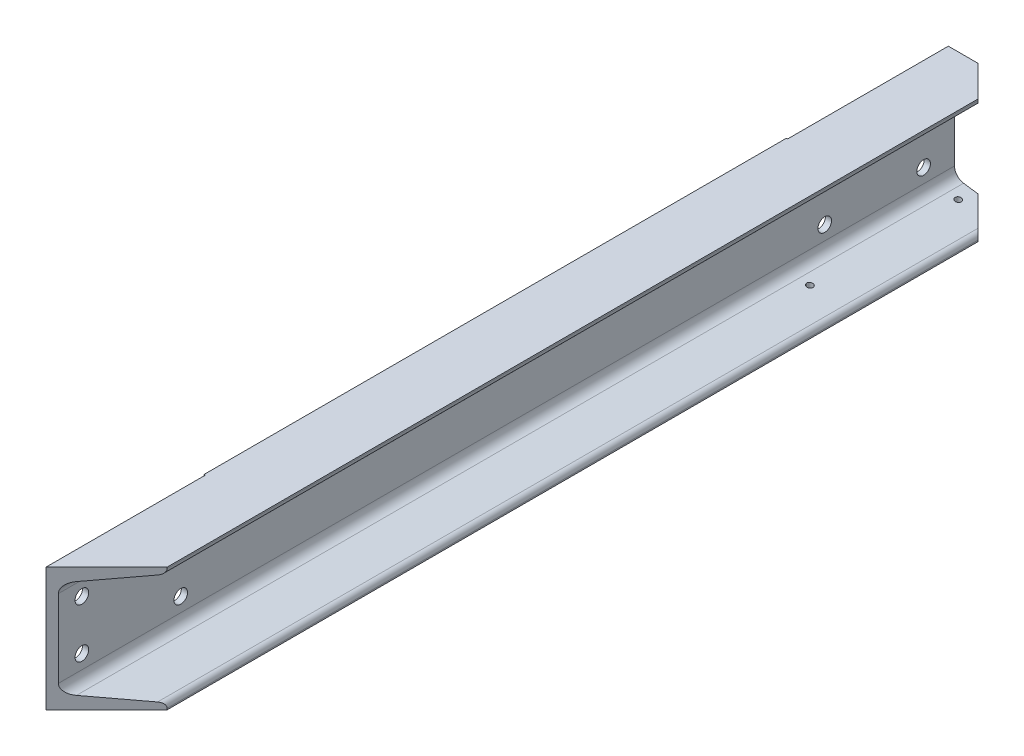
SolidWorks part; units mm, degrees
material "1023 carbon steel plate (SS)"
ref_plane "Front Plane" through (0, 0, 0) normal (0, 0, 1) x (1, 0, 0)
ref_plane "Top Plane" through (0, 0, 0) normal (0, 1, 0) x (1, 0, 0)
ref_plane "Right Plane" through (0, 0, 0) normal (1, 0, 0) x (0, 0, -1)
sketch "Sketch1" plane through (0, 0, 0) normal (0, 0, 1) x (1, 0, 0)
  line L0 (0, 0) -> (0, -100)
  line L1 (0, -100) -> (50, -100)
  line L2 (0, 0) -> (50, 0)
  line L3 (50, 0) -> (50, -1.0747)
  line L4 (50, -100) -> (50, -98.9253)
  line L5 (46.1263, -5.5309) -> (13.317, -10.1419)
  line L6 (6, -18.5592) -> (6, -81.4408)
  line L7 (13.317, -89.8581) -> (46.1263, -94.4691)
  line L8 (25, 0) -> (25, -8.5) construction
  line L9 (25, -100) -> (25, -91.5) construction
  arc A0 (6, -81.4408) -> (13.317, -89.8581) centre (14.5, -81.4408) ccw
  arc A1 (13.317, -10.1419) -> (6, -18.5592) centre (14.5, -18.5592) ccw
  arc A2 (50, -98.9253) -> (46.1263, -94.4691) centre (45.5, -98.9253) ccw
  arc A3 (50, -1.0747) -> (46.1263, -5.5309) centre (45.5, -1.0747) cw
  dimension "D8" = 8.5
  dimension "D9" = 4.5
  dimension "D1" = 100
  dimension "D2" = 50
  dimension "D3" = 50
  dimension "D4" = 6
  dimension "D5" = 8.5
  dimension "D6" = 8.5
  dimension "D7" = 98
extrude "Boss-Extrude1" add sketch "Sketch1" along normal blind 750
sketch "Sketch2" plane through (0, 0, 0) normal (0, 1, 0) x (1, 0, 0)
  line L0 (258.9926, -472.0074) -> (0, -731)
  line L2 (45.0448, -785.8728) -> (459.457, -587.6756)
  line L3 (459.457, -587.6756) -> (258.9926, -472.0074)
  line L4 (0, -750) -> (0, 0) construction
  line L5 (0, -731) -> (-59.7772, -772.2622)
  line L6 (-59.7772, -772.2622) -> (30.8414, -818.1599)
  line L7 (30.8414, -818.1599) -> (45.0448, -785.8728)
  line L8 (25, 0) -> (50, -25)
  line L9 (50, 0) -> (0, 0) construction
  line L10 (50, -750) -> (50, 0) construction
  line L11 (50, -25) -> (50, 48.4172)
  line L12 (50, 48.4172) -> (25, 0)
  dimension "D1" = 45
  dimension "D2" = 731
  dimension "D3" = 25
  dimension "D4" = 25
extrude "Cut-Extrude1" cut sketch "Sketch2" against normal blind 730
sketch "Sketch3" plane through (0, 0, 0) normal (-1, 0, 0) x (0, 0, 1)
  line L0 (130, 38.7018) -> (130, -162.7252)
  line L1 (130, -162.7252) -> (-125.6336, -119.6063)
  line L2 (-125.6336, -119.6063) -> (-100.4183, 29.8844)
  line L3 (-100.4183, 29.8844) -> (130, 38.7018)
  line L4 (0, 0) -> (0, -100) construction
  line L5 (731, -100) -> (731, 0) construction
  line L6 (847.7925, 272.7759) -> (601, 272.7759)
  line L7 (847.7925, 272.7759) -> (847.7925, -138.7018)
  line L8 (847.7925, -138.7018) -> (601, -138.7018)
  line L9 (601, 272.7759) -> (601, -138.7018)
  line L10 (847.7925, 272.7759) -> (601, -138.7018) construction
  line L11 (847.7925, -138.7018) -> (601, 272.7759) construction
  point P6 (724.3962, 67.0371)
  dimension "D1" = 130
  dimension "D2" = 130
extrude "Cut-Extrude2" cut sketch "Sketch3" against normal blind 1
sketch "Sketch4" plane through (1, 0, 0) normal (-1, 0, 0) x (0, 0, 1)
  line L0 (0, 0) -> (0, -100) construction
  line L1 (0, 0) -> (130, 0) construction
  line L2 (365.5, 0) -> (365.5, -47.3528) construction
  line L3 (601, 0) -> (130, 0) construction
  circle A0 centre (25, -30) radius 5.5
  circle A1 centre (105, -30) radius 5.5
  circle A2 centre (25, -70) radius 5.5
  circle A3 centre (105, -70) radius 5.5
  circle A4 centre (626, -30) radius 5.5
  circle A5 centre (706, -70) radius 5.5
  circle A6 centre (626, -70) radius 5.5
  circle A7 centre (706, -30) radius 5.5
  point P14 (0, -50)
  point P17 (65, 0)
  dimension "D5" = 11
  dimension "D1" = 40
  dimension "D2" = 80
  dimension "D3" = 20
  dimension "D4" = 40
extrude "Cut-Extrude3" cut sketch "Sketch4" against normal blind 10
sketch "Sketch5" plane through (0, -100, 0) normal (0, -1, 0) x (1, 0, 0)
  line L0 (1, 130) -> (1, 0) construction
  line L1 (1, 0) -> (25, 0) construction
  circle A0 centre (21.5, 12.5) radius 2
  circle A1 centre (21.5, 132.5) radius 2
  dimension "D1" = 4
  dimension "D4" = 120
  dimension "D2" = 20.5
  dimension "D3" = 12.5
hole_wizard "M6 Tapped Hole1" positions "Sketch6" profile "Sketch7" tap size "M6" standard "ISO"
sketch "Sketch6" plane through (0, -100, 0) normal (0, -1, 0) x (-1, 0, 0)
  point P0 (-21.5, -12.5)
sketch "Sketch7" plane through (21.5, -100, 12.5) normal (1, 0, 0) x (0, 0, -1)
  line L0 (0, 0) -> (0, 16.5022)
  line L1 (0, 16.5022) -> (2.5, 15)
  line L2 (2.5, 15) -> (2.5, 0)
  line L5 (2.5, 0) -> (0, 0)
  line L10 (0, 16.5022) -> (-2.5, 15) construction
  line L11 (0, -6.35) -> (0, 107.95) construction
  dimension "螺纹孔钻头直径" = 5
  dimension "螺纹孔钻头深度" = 15
  dimension "导头角度" = 118
cosmetic thread "Cosmetic thread 1" parameters "D1"=12, "D2"=6
hole_wizard "M6 Tapped Hole2" positions "Sketch8" profile "Sketch9" tap size "M6" standard "ISO"
sketch "Sketch8" plane through (0, -100, 0) normal (0, -1, 0) x (-1, 0, 0)
  point P0 (-21.5, -132.5)
sketch "Sketch9" plane through (21.5, -100, 132.5) normal (1, 0, 0) x (0, 0, -1)
  line L0 (0, 0) -> (0, 16.5022)
  line L1 (0, 16.5022) -> (2.5, 15)
  line L2 (2.5, 15) -> (2.5, 0)
  line L5 (2.5, 0) -> (0, 0)
  line L10 (0, 16.5022) -> (-2.5, 15) construction
  line L11 (0, -6.35) -> (0, 107.95) construction
  dimension "螺纹孔钻头直径" = 5
  dimension "螺纹孔钻头深度" = 15
  dimension "导头角度" = 118
cosmetic thread "Cosmetic thread 2" parameters "D1"=12, "D2"=6
